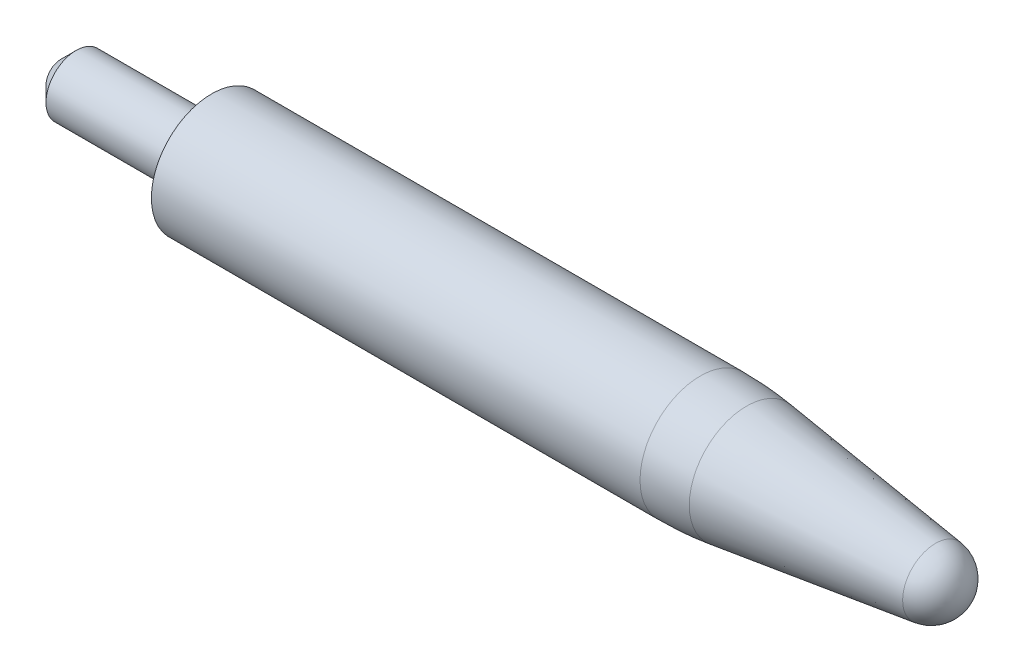
from build123d import *

# Parameters (mm, degrees)
SKETCH2_R           = 1
BOSS_EXTRUDE1_DEPTH = 5
CHAMFER1_SIZE       = 0.5


with BuildPart() as part:
    # Sketch1 → Revolve1 (revolve)
    with BuildSketch(Plane.XY, mode=Mode.PRIVATE) as revolve1_sk:
        with BuildLine():
            Line((0, 0), (0, 2))
            Line((0, 2), (16.22853262, 2))
            ThreePointArc((16.22853262, 2), (16.998410661, 1.975278193), (17.765116572, 1.901214634))
            Line((17.765116572, 1.901214634), (24.040853529, 1.090944675))
            ThreePointArc((24.040853529, 1.090944675), (24.726117087, 0.72631299), (25, 0))
            Line((25, 0), (0, 0))
        make_face()
    revolve(revolve1_sk.sketch.rotate(Axis((0, 0, 0), (1, 0, 0)), 90), axis=Axis((0, 0, 0), (1, 0, 0)))

    # Sketch2 → Boss-Extrude1 (add)
    with BuildSketch(Plane.ZY):
        Circle(SKETCH2_R)
    extrude(amount=BOSS_EXTRUDE1_DEPTH)

    # Chamfer1
    chamfer1_edges = [part.edges().sort_by_distance(p)[0] for p in [
        (-5, 0, -1),
    ]]
    chamfer(chamfer1_edges, length=CHAMFER1_SIZE)


solid = part.part
